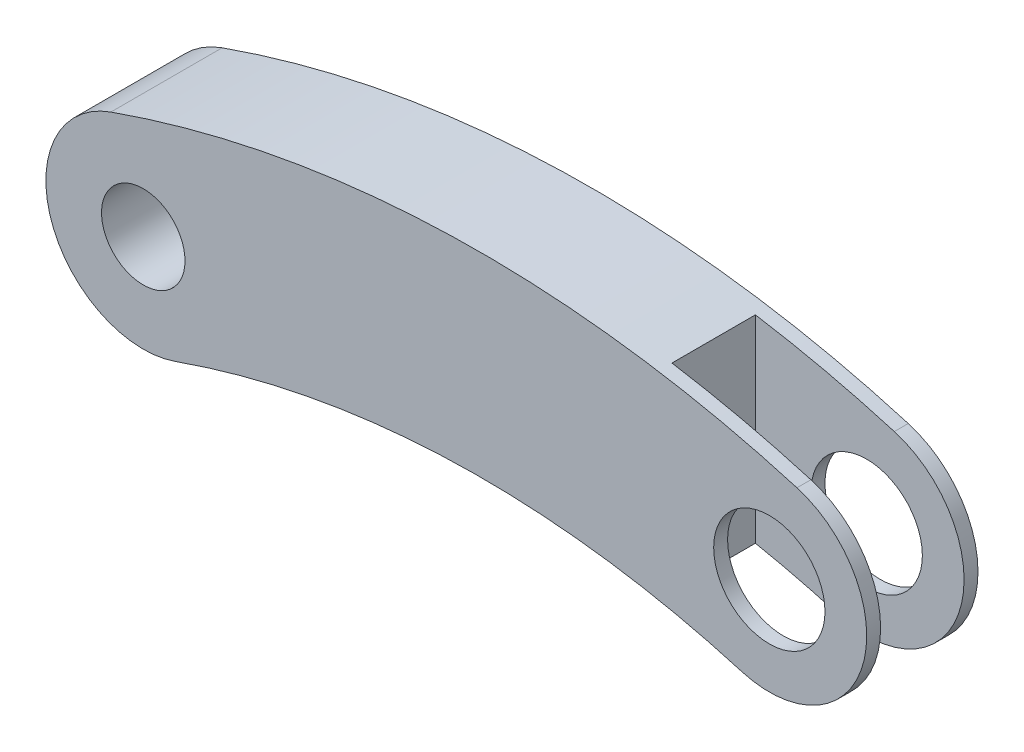
SolidWorks part; units mm, degrees
material "1060 Alloy"
ref_plane "Front Plane" through (0, 0, 0) normal (0, 0, 1) x (1, 0, 0)
ref_plane "Top Plane" through (0, 0, 0) normal (0, 1, 0) x (1, 0, 0)
ref_plane "Right Plane" through (0, 0, 0) normal (1, 0, 0) x (0, 0, -1)
sketch "Sketch1" plane through (0, 0, 0) normal (0, 0, 1) x (1, 0, 0)
  arc A0 (-50.7579, -0.0488) -> (-1.4429, 1.2191) centre (-24.1445, -75.4923) cw
  arc A1 (-46.1006, -13.2514) -> (-5.4157, -12.2054) centre (-24.1445, -75.4923) cw
  arc A2 (-5.4157, -12.2054) -> (-1.4429, 1.2191) centre (-3.4293, -5.4932) ccw
  arc A3 (-50.7579, -0.0488) -> (-46.1006, -13.2514) centre (-48.4293, -6.6501) ccw
  circle A4 centre (-48.4293, -6.6501) radius 3
  circle A5 centre (-3.4293, -5.4932) radius 4
  dimension "D1" = 80
  dimension "D3" = 8
  dimension "D4" = 6
  dimension "D6" = 14
  dimension "D7" = 6
  dimension "D8" = 8
  dimension "D9" = 14
  dimension "D5" = 45
  dimension "D2" = 14
extrude "Boss-Extrude1" add sketch "Sketch1" along normal blind 8
sketch "Sketch2" plane through (0, 0, 0) normal (0, 1, 0) x (1, 0, 0)
  line L0 (3.5707, -8) -> (3.5707, 0) construction
  line L1 (-11.4293, -1) -> (18.5707, -1)
  line L2 (-11.4293, -1) -> (-11.4293, -7)
  line L3 (-11.4293, -7) -> (18.5707, -7)
  line L4 (18.5707, -1) -> (18.5707, -7)
  line L5 (-11.4293, -1) -> (18.5707, -7) construction
  line L6 (-11.4293, -7) -> (18.5707, -1) construction
  point P0 (3.5707, -4)
  dimension "D1" = 6
  dimension "D2" = 30
extrude "Cut-Extrude1" cut sketch "Sketch2" against normal blind 16 and the other way blind 8
scale "Scale1" scale about origin uniform scaling yes scale factor 0.5
